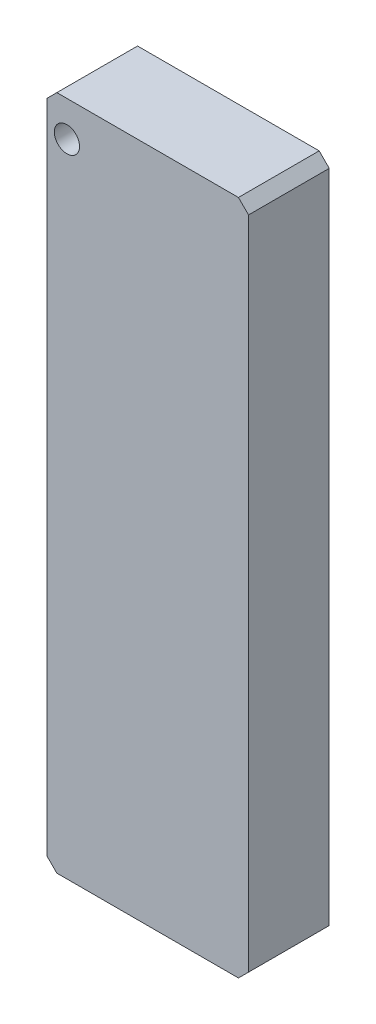
from build123d import *

# Parameters (mm, degrees)
SKETCH_1_W             = 20
SKETCH_1_H             = 67
EXTRUDE_1_DEPTH        = 4
HOLE_WIZARD_M3_1_D     = 2.5
HOLE_WIZARD_M4_1_D     = 3.3
HOLE_WIZARD_M4_1_DEPTH = 10.1
HOLE_WIZARD_M4_1_TIP   = 0.991420021
CHAMFER_1_SIZE         = 1


with BuildPart() as part:
    # 草图1 → 凸台-拉伸1 (new, symmetric)
    with BuildSketch(Plane.XY):
        Rectangle(SKETCH_1_W, SKETCH_1_H)
    extrude(amount=EXTRUDE_1_DEPTH, both=True)

    # M3 螺纹孔1 (through all)
    with Locations(Plane(origin=(0, 0, -4), x_dir=(-1, 0, 0), z_dir=(0, 0, -1))):
        with Locations((8, 30)):
            Hole(HOLE_WIZARD_M3_1_D / 2)

    # M4 螺纹孔1
    with Locations(Plane(origin=(0, -33.5, 0), x_dir=(-1, 0, 0), z_dir=(0, -1, 0))):
        with Locations((6, 0), (-6, 0)):
            Hole(HOLE_WIZARD_M4_1_D / 2, depth=HOLE_WIZARD_M4_1_DEPTH)
            with Locations((0, 0, -(HOLE_WIZARD_M4_1_DEPTH + HOLE_WIZARD_M4_1_TIP / 2))):  # 118° drill point
                Cone(0, HOLE_WIZARD_M4_1_D / 2, HOLE_WIZARD_M4_1_TIP, mode=Mode.SUBTRACT)

    # 倒角1
    chamfer_1_edges = [part.edges().sort_by_distance(p)[0] for p in [
        (10, -33.5, 0),
        (-10, -33.5, 0),
        (-10, 33.5, 0),
        (10, 33.5, 0),
    ]]
    chamfer(chamfer_1_edges, length=CHAMFER_1_SIZE)


solid = part.part
